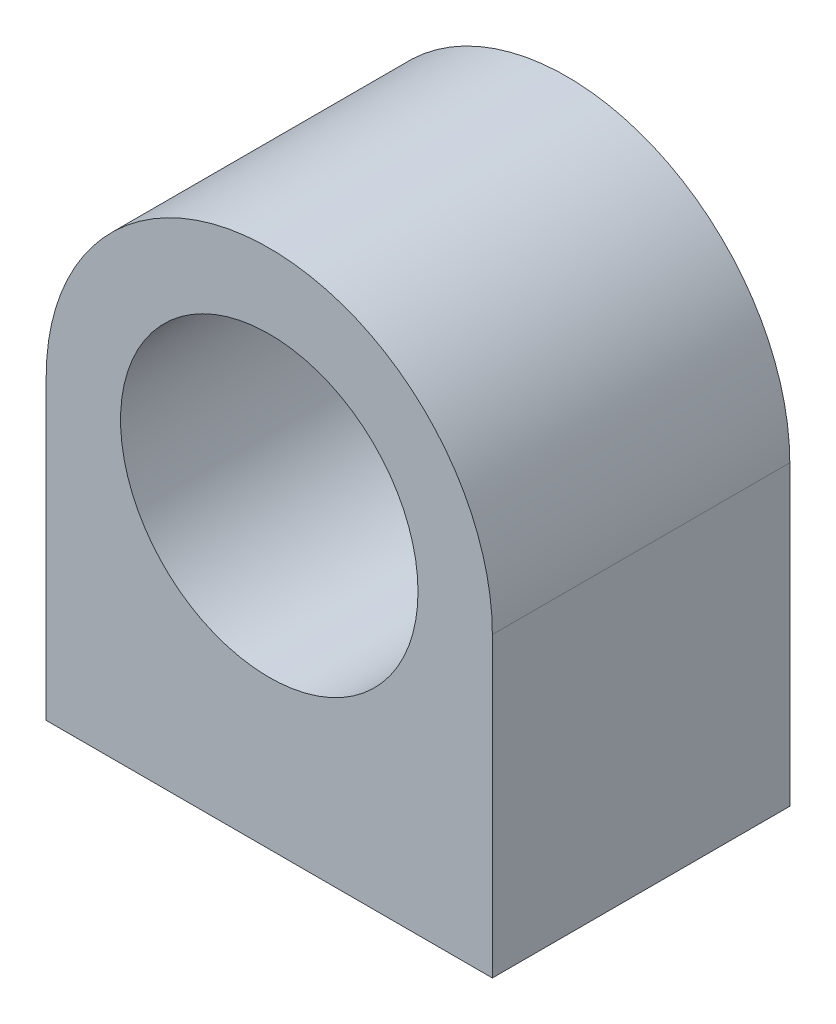
from build123d import *

# Parameters (mm, degrees)
SKETCH_1_R      = 5
EXTRUDE_1_DEPTH = 10


with BuildPart() as part:
    # 草图1 → 凸台-拉伸1 (new body)
    with BuildSketch(Plane.XY):
        with BuildLine():
            Line((7.5, 0), (7.5, -10))
            Line((7.5, -10), (-7.5, -10))
            Line((-7.5, -10), (-7.5, 0))
            ThreePointArc((-7.5, 0), (0, 7.5), (7.5, 0))
        make_face()
        Circle(SKETCH_1_R, mode=Mode.SUBTRACT)
    extrude(amount=EXTRUDE_1_DEPTH)


solid = part.part
